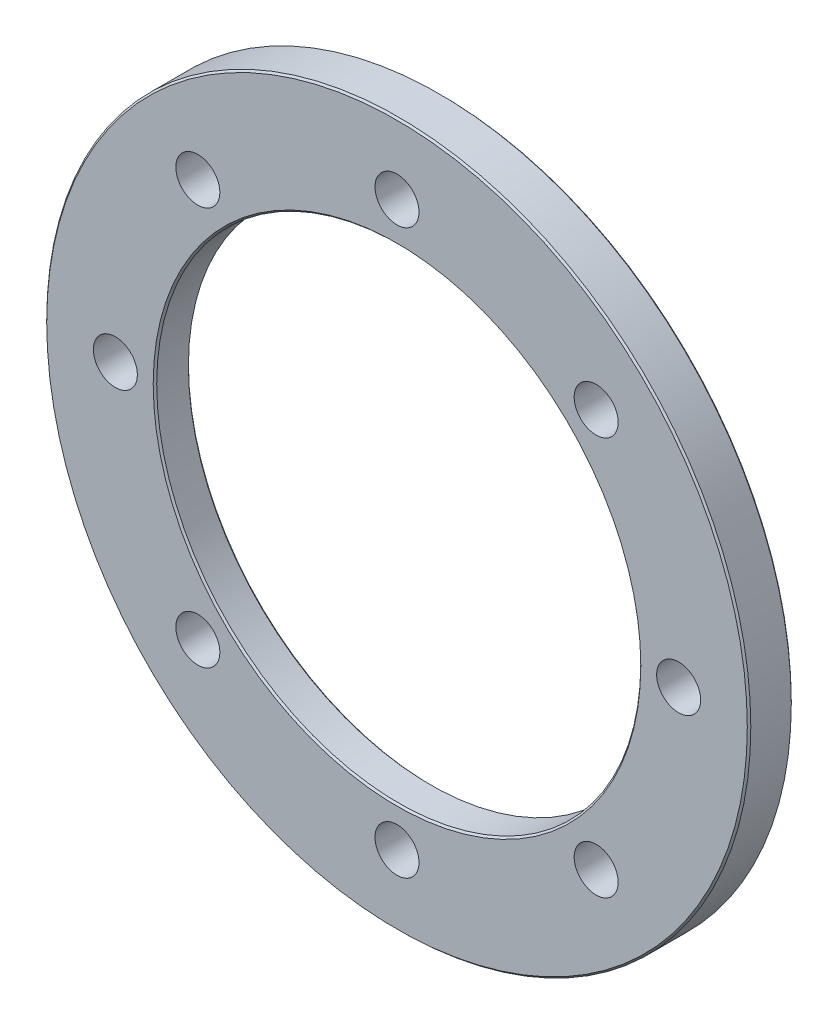
from build123d import *

# Parameters (mm, degrees)
SKETCH1_R           = 200
SKETCH1_R_2         = 137.5
SKETCH1_R_3         = 12.5
BOSS_EXTRUDE1_DEPTH = 25
CHAMFER1_SIZE       = 1
SKETCH4_R           = 177.5
CUT_EXTRUDE2_DEPTH  = 5
FILLET1_R           = 2
CHAMFER2_SIZE       = 1


with BuildPart() as part:
    # Sketch1 → Boss-Extrude1 (new body)
    with BuildSketch(Plane.XY):
        Circle(SKETCH1_R)
        Circle(SKETCH1_R_2, mode=Mode.SUBTRACT)
        with Locations((0, 160)):
            Circle(SKETCH1_R_3, mode=Mode.SUBTRACT)
        with Locations((113.13708499, 113.13708499)):
            Circle(SKETCH1_R_3, mode=Mode.SUBTRACT)
        with Locations((160, 0)):
            Circle(SKETCH1_R_3, mode=Mode.SUBTRACT)
        with Locations((113.13708499, -113.13708499)):
            Circle(SKETCH1_R_3, mode=Mode.SUBTRACT)
        with Locations((0, -160)):
            Circle(SKETCH1_R_3, mode=Mode.SUBTRACT)
        with Locations((-113.13708499, -113.13708499)):
            Circle(SKETCH1_R_3, mode=Mode.SUBTRACT)
        with Locations((-160, 0)):
            Circle(SKETCH1_R_3, mode=Mode.SUBTRACT)
        with Locations((-113.13708499, 113.13708499)):
            Circle(SKETCH1_R_3, mode=Mode.SUBTRACT)
    extrude(amount=BOSS_EXTRUDE1_DEPTH)

    # Chamfer1
    chamfer1_edges = [part.edges().sort_by_distance(p)[0] for p in [
        (-200, 0, 0),
        (-200, 0, 25),
        (-137.5, 0, 0),
        (-137.5, 0, 25),
    ]]
    chamfer(chamfer1_edges, length=CHAMFER1_SIZE)

    # Sketch4 → Cut-Extrude2 (cut)
    with BuildSketch(Plane(origin=(0, 0, 0), x_dir=(-1, 0, 0), z_dir=(0, 0, -1))):
        Circle(SKETCH4_R)
    extrude(amount=-CUT_EXTRUDE2_DEPTH, mode=Mode.SUBTRACT)

    # Fillet1
    fillet1_edges = [part.edges().sort_by_distance(p)[0] for p in [
        (177.5, 0, 5),
    ]]
    fillet(fillet1_edges, radius=FILLET1_R)

    # Chamfer2
    chamfer2_edges = [part.edges().sort_by_distance(p)[0] for p in [
        (-137.5, 0, 5),
        (177.5, 0, 0),
    ]]
    chamfer(chamfer2_edges, length=CHAMFER2_SIZE)


solid = part.part
